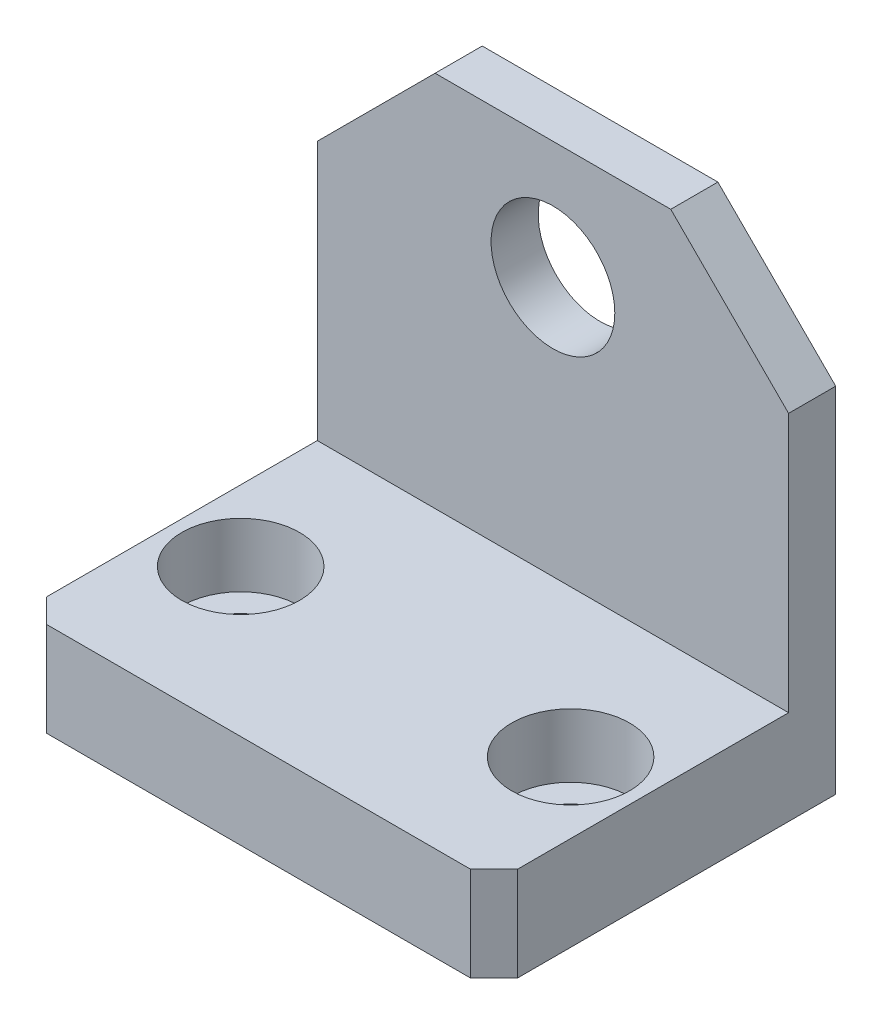
SolidWorks part; units mm, degrees
material "SS41"
ref_plane "Front Plane" through (0, 0, 0) normal (0, 0, 1) x (1, 0, 0)
ref_plane "Top Plane" through (0, 0, 0) normal (0, 1, 0) x (1, 0, 0)
ref_plane "Right Plane" through (0, 0, 0) normal (1, 0, 0) x (0, 0, -1)
sketch "Sketch2" plane through (0, 0, 0) normal (0, 0, 1) x (1, 0, 0)
  line L1 (-20, 20) -> (20, 20)
  line L2 (-20, 20) -> (-20, -20)
  line L3 (-20, -20) -> (20, -20)
  line L4 (20, 20) -> (20, -20)
  line L5 (-20, 20) -> (20, -20) construction
  line L6 (-20, -20) -> (20, 20) construction
  point P0 (0, 0)
  dimension "D1" = 40
  dimension "D2" = 40
extrude "Boss-Extrude1" add sketch "Sketch2" along normal blind 4
sketch "Sketch3" plane through (0, 0, 4) normal (0, 0, 1) x (1, 0, 0)
  line L0 (20, -20) -> (20, 20) construction
  line L1 (-20, -20) -> (20, -20)
  line L2 (-20, -20) -> (-20, -12)
  line L3 (-20, -12) -> (20, -12)
  line L4 (20, -20) -> (20, -12)
  dimension "D1" = 8
extrude "Boss-Extrude2" add sketch "Sketch3" along normal blind 25
sketch "Sketch4" plane through (0, 0, 4) normal (0, 0, 1) x (1, 0, 0)
  line L0 (0, 20) -> (0, 0) construction
  line L1 (20, 20) -> (-20, 20) construction
  line L2 (-20, -20) -> (20, -20) construction
  circle A0 centre (0, 10) radius 5.25
  dimension "D1" = 30
  dimension "D2" = 10.5
extrude "Cut-Extrude1" cut sketch "Sketch4" against normal blind 25
chamfer "Chamfer1" distance 10 angle 45 2 edges at (20, 20, 2) (-20, 20, 2)
hole_wizard "CBORE for M5 Hex Socket Head Cap Screw1" positions "Sketch6" profile "Sketch5" counterbore size "M5" standard "Iso" end condition through all
sketch "Sketch6" plane through (0, -12, 0) normal (0, 1, 0) x (1, 0, 0)
  line L0 (0, -29) -> (0, 0) construction
  line L1 (20, -29) -> (-20, -29) construction
  point P0 (-14, -16.5)
  point P2 (14, -16.5)
  dimension "D1" = 12.5
  dimension "D2" = 28
sketch "Sketch5" plane through (-14, -12, 16.5) normal (1, 0, 0) x (0, 0, 1)
  line L0 (0, 0) -> (0, 8)
  line L1 (0, 8) -> (2.75, 8)
  line L3 (2.75, 8) -> (2.75, 5.4)
  line L4 (2.75, 5.4) -> (5, 5.4)
  line L5 (5, 5.4) -> (5, 0)
  line L7 (5, 0) -> (0, 0)
  line L11 (0, -6.35) -> (0, 107.95) construction
  dimension "通孔孔直径" = 5.5
  dimension "通孔孔深度" = 8
  dimension "柱形沉头孔直径" = 10
  dimension "柱形沉头孔深度" = 5.4
chamfer "Chamfer2" distance 2 angle 45 2 edges at (20, -16, 29) (-20, -16, 29)
